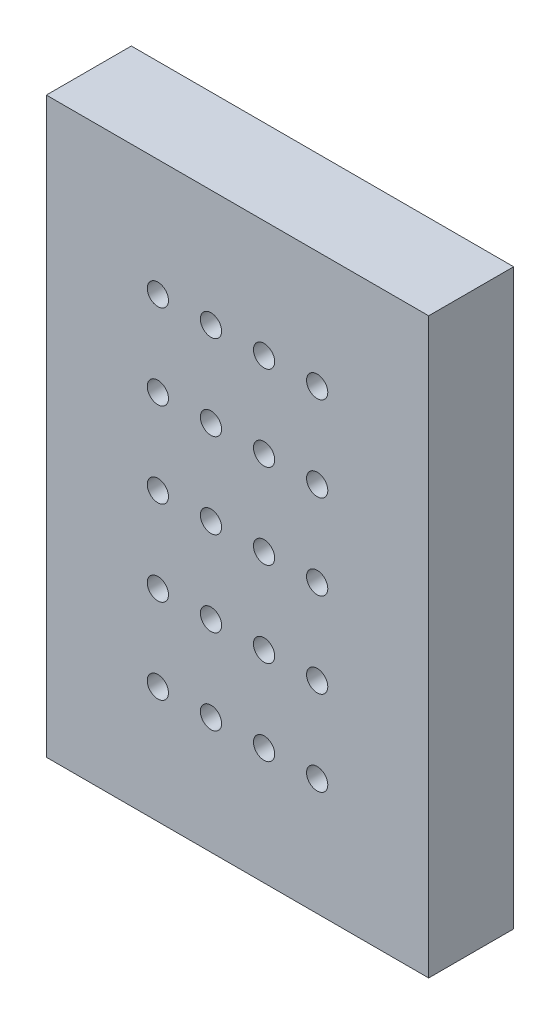
from build123d import *

# Parameters (mm, degrees)
SKETCH_1_W               = 18
SKETCH_1_H               = 27
EXTRUDE_1_DEPTH          = 4
CUT_EXTRUDE_1_REACH      = 18.711
SKETCH_2_R               = 0.5
PATTERN_LINEAR_2_COUNT   = 3
PATTERN_LINEAR_2_PITCH   = 4
MIRROR_1_COPY_1_REACH    = 18.711
MIRROR_1_COPY_1_SKETCH_R = 0.5
MIRROR_1_COPY_2_REACH    = 18.711
MIRROR_1_COPY_2_SKETCH_R = 0.5


with BuildPart() as part:
    # 草图1 → 凸台-拉伸1 (new body)
    with BuildSketch(Plane.XY):
        Rectangle(SKETCH_1_W, SKETCH_1_H)
    extrude(amount=EXTRUDE_1_DEPTH)

    # 草图2 → 切除-拉伸1 (cut, up to next)
    with BuildSketch(Plane.XY.offset(4), mode=Mode.PRIVATE) as cut_extrude_1_sk1:
        with Locations((-1.25, 0)):
            Circle(SKETCH_2_R)
    cut_extrude_1_tool1 = extrude(cut_extrude_1_sk1.sketch, amount=-CUT_EXTRUDE_1_REACH, mode=Mode.PRIVATE) & part.part
    # 草图2 → 切除-拉伸1 (cut, up to next)
    with BuildSketch(Plane.XY.offset(4), mode=Mode.PRIVATE) as cut_extrude_1_sk2:
        with Locations((-3.75, 0)):
            Circle(SKETCH_2_R)
    cut_extrude_1_tool2 = extrude(cut_extrude_1_sk2.sketch, amount=-CUT_EXTRUDE_1_REACH, mode=Mode.PRIVATE) & part.part
    # 草图2 → 切除-拉伸1 (cut, up to next)
    with BuildSketch(Plane.XY.offset(4), mode=Mode.PRIVATE) as cut_extrude_1_sk3:
        with Locations((1.25, 0)):
            Circle(SKETCH_2_R)
    cut_extrude_1_tool3 = extrude(cut_extrude_1_sk3.sketch, amount=-CUT_EXTRUDE_1_REACH, mode=Mode.PRIVATE) & part.part
    # 草图2 → 切除-拉伸1 (cut, up to next)
    with BuildSketch(Plane.XY.offset(4), mode=Mode.PRIVATE) as cut_extrude_1_sk4:
        with Locations((3.75, 0)):
            Circle(SKETCH_2_R)
    cut_extrude_1_tool4 = extrude(cut_extrude_1_sk4.sketch, amount=-CUT_EXTRUDE_1_REACH, mode=Mode.PRIVATE) & part.part
    cut_extrude_1_1 = cut_extrude_1_tool1.solids().sort_by_distance((-1.25, 0, 4))[0]
    add(cut_extrude_1_1, mode=Mode.SUBTRACT)
    cut_extrude_1_2 = cut_extrude_1_tool2.solids().sort_by_distance((-3.75, 0, 4))[0]
    add(cut_extrude_1_2, mode=Mode.SUBTRACT)
    cut_extrude_1_3 = cut_extrude_1_tool3.solids().sort_by_distance((1.25, 0, 4))[0]
    add(cut_extrude_1_3, mode=Mode.SUBTRACT)
    cut_extrude_1_4 = cut_extrude_1_tool4.solids().sort_by_distance((3.75, 0, 4))[0]
    add(cut_extrude_1_4, mode=Mode.SUBTRACT)
    cut_extrude_1 = cut_extrude_1_1 + cut_extrude_1_2 + cut_extrude_1_3 + cut_extrude_1_4  # 切除-拉伸1 as one shape, for the pattern or mirror that repeats it

    # 阵列(线性)2: 切除-拉伸1 ×3
    with Locations(*[(0, -i * PATTERN_LINEAR_2_PITCH, 0) for i in range(1, PATTERN_LINEAR_2_COUNT)]):
        add(cut_extrude_1, mode=Mode.SUBTRACT)

    # 镜向1 copy 1 sketch → 镜向1 copy 1 (cut, up to next)
    with BuildSketch(Plane(origin=(0, 4, 4), x_dir=(1, 0, 0), z_dir=(0, 0, 1)), mode=Mode.PRIVATE) as mirror_1_copy_1_sk1:
        with Locations((-1.25, 0)):
            Circle(MIRROR_1_COPY_1_SKETCH_R)
    mirror_1_copy_1_tool1 = extrude(mirror_1_copy_1_sk1.sketch, amount=-MIRROR_1_COPY_1_REACH, mode=Mode.PRIVATE) & part.part
    # 镜向1 copy 1 sketch → 镜向1 copy 1 (cut, up to next)
    with BuildSketch(Plane(origin=(0, 4, 4), x_dir=(1, 0, 0), z_dir=(0, 0, 1)), mode=Mode.PRIVATE) as mirror_1_copy_1_sk2:
        with Locations((-3.75, 0)):
            Circle(MIRROR_1_COPY_1_SKETCH_R)
    mirror_1_copy_1_tool2 = extrude(mirror_1_copy_1_sk2.sketch, amount=-MIRROR_1_COPY_1_REACH, mode=Mode.PRIVATE) & part.part
    # 镜向1 copy 1 sketch → 镜向1 copy 1 (cut, up to next)
    with BuildSketch(Plane(origin=(0, 4, 4), x_dir=(1, 0, 0), z_dir=(0, 0, 1)), mode=Mode.PRIVATE) as mirror_1_copy_1_sk3:
        with Locations((1.25, 0)):
            Circle(MIRROR_1_COPY_1_SKETCH_R)
    mirror_1_copy_1_tool3 = extrude(mirror_1_copy_1_sk3.sketch, amount=-MIRROR_1_COPY_1_REACH, mode=Mode.PRIVATE) & part.part
    # 镜向1 copy 1 sketch → 镜向1 copy 1 (cut, up to next)
    with BuildSketch(Plane(origin=(0, 4, 4), x_dir=(1, 0, 0), z_dir=(0, 0, 1)), mode=Mode.PRIVATE) as mirror_1_copy_1_sk4:
        with Locations((3.75, 0)):
            Circle(MIRROR_1_COPY_1_SKETCH_R)
    mirror_1_copy_1_tool4 = extrude(mirror_1_copy_1_sk4.sketch, amount=-MIRROR_1_COPY_1_REACH, mode=Mode.PRIVATE) & part.part
    add(mirror_1_copy_1_tool1.solids().sort_by_distance((-1.25, 4, 4))[0], mode=Mode.SUBTRACT)
    add(mirror_1_copy_1_tool2.solids().sort_by_distance((-3.75, 4, 4))[0], mode=Mode.SUBTRACT)
    add(mirror_1_copy_1_tool3.solids().sort_by_distance((1.25, 4, 4))[0], mode=Mode.SUBTRACT)
    add(mirror_1_copy_1_tool4.solids().sort_by_distance((3.75, 4, 4))[0], mode=Mode.SUBTRACT)

    # 镜向1 copy 2 sketch → 镜向1 copy 2 (cut, up to next)
    with BuildSketch(Plane(origin=(0, 8, 4), x_dir=(1, 0, 0), z_dir=(0, 0, 1)), mode=Mode.PRIVATE) as mirror_1_copy_2_sk1:
        with Locations((-1.25, 0)):
            Circle(MIRROR_1_COPY_2_SKETCH_R)
    mirror_1_copy_2_tool1 = extrude(mirror_1_copy_2_sk1.sketch, amount=-MIRROR_1_COPY_2_REACH, mode=Mode.PRIVATE) & part.part
    # 镜向1 copy 2 sketch → 镜向1 copy 2 (cut, up to next)
    with BuildSketch(Plane(origin=(0, 8, 4), x_dir=(1, 0, 0), z_dir=(0, 0, 1)), mode=Mode.PRIVATE) as mirror_1_copy_2_sk2:
        with Locations((-3.75, 0)):
            Circle(MIRROR_1_COPY_2_SKETCH_R)
    mirror_1_copy_2_tool2 = extrude(mirror_1_copy_2_sk2.sketch, amount=-MIRROR_1_COPY_2_REACH, mode=Mode.PRIVATE) & part.part
    # 镜向1 copy 2 sketch → 镜向1 copy 2 (cut, up to next)
    with BuildSketch(Plane(origin=(0, 8, 4), x_dir=(1, 0, 0), z_dir=(0, 0, 1)), mode=Mode.PRIVATE) as mirror_1_copy_2_sk3:
        with Locations((1.25, 0)):
            Circle(MIRROR_1_COPY_2_SKETCH_R)
    mirror_1_copy_2_tool3 = extrude(mirror_1_copy_2_sk3.sketch, amount=-MIRROR_1_COPY_2_REACH, mode=Mode.PRIVATE) & part.part
    # 镜向1 copy 2 sketch → 镜向1 copy 2 (cut, up to next)
    with BuildSketch(Plane(origin=(0, 8, 4), x_dir=(1, 0, 0), z_dir=(0, 0, 1)), mode=Mode.PRIVATE) as mirror_1_copy_2_sk4:
        with Locations((3.75, 0)):
            Circle(MIRROR_1_COPY_2_SKETCH_R)
    mirror_1_copy_2_tool4 = extrude(mirror_1_copy_2_sk4.sketch, amount=-MIRROR_1_COPY_2_REACH, mode=Mode.PRIVATE) & part.part
    add(mirror_1_copy_2_tool1.solids().sort_by_distance((-1.25, 8, 4))[0], mode=Mode.SUBTRACT)
    add(mirror_1_copy_2_tool2.solids().sort_by_distance((-3.75, 8, 4))[0], mode=Mode.SUBTRACT)
    add(mirror_1_copy_2_tool3.solids().sort_by_distance((1.25, 8, 4))[0], mode=Mode.SUBTRACT)
    add(mirror_1_copy_2_tool4.solids().sort_by_distance((3.75, 8, 4))[0], mode=Mode.SUBTRACT)


solid = part.part
